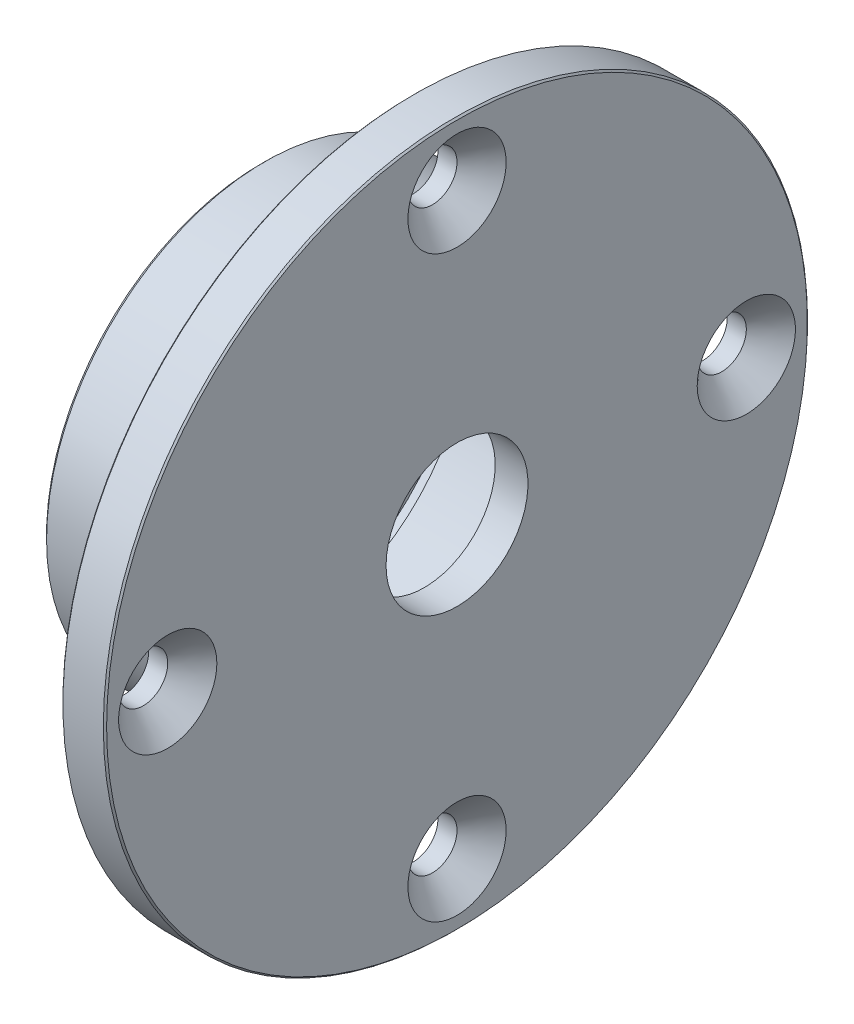
SolidWorks part; units mm, degrees
material "6063-T6"
ref_plane "Front Plane" through (0, 0, 0) normal (0, 0, 1) x (1, 0, 0)
ref_plane "Top Plane" through (0, 0, 0) normal (0, 1, 0) x (1, 0, 0)
ref_plane "Right Plane" through (0, 0, 0) normal (1, 0, 0) x (0, 0, -1)
sketch "Sketch1" plane through (0, 0, 0) normal (0, 0, 1) x (1, 0, 0)
  line L0 (0, 16) -> (1.6954, 16)
  line L1 (13, 16) -> (13, 12.5)
  line L2 (13, 12.5) -> (15, 12.5)
  line L3 (15, 12.5) -> (15, 0)
  line L4 (15, 0) -> (18, 0)
  line L5 (18, 0) -> (18, 32.5)
  line L6 (18, 32.5) -> (14, 32.5)
  line L7 (14, 32.5) -> (14, 20)
  line L8 (14, 20) -> (0, 20)
  line L9 (0, 20) -> (0, 16)
  line L10 (1.6954, 16) -> (1.6954, 16.85)
  line L11 (1.6954, 16.85) -> (2.9954, 16.85)
  line L12 (2.9954, 16.85) -> (2.9954, 16)
  line L13 (2.9954, 16) -> (13, 16)
  dimension "D1" = 16
  dimension "D2" = 2
  dimension "D3" = 12.5
  dimension "D4" = 18
  dimension "D5" = 4
  dimension "D6" = 3
  dimension "D7" = 20
  dimension "D8" = 32.5
  dimension "D9" = 1.3
  dimension "D10" = 16.85
  dimension "D11" = 10.0046
revolve "Revolve1" add sketch "Sketch1" angle 360 about L4
sketch "Sketch2" plane through (0, 0, 0) normal (0, 1, 0) x (1, 0, 0)
  line L0 (14, 26.5) -> (18, 26.5)
  line L1 (14, 32.5) -> (14, -32.5) construction
  line L2 (18, -32.5) -> (18, 32.5) construction
  line L3 (18, 26.5) -> (18, 31)
  line L4 (18, 31) -> (15.75, 28.75)
  line L5 (15.75, 28.75) -> (14, 28.75)
  line L6 (14, 28.75) -> (14, 26.5)
  dimension "D1" = 26.5
  dimension "D2" = 2.25
  dimension "D3" = 4.5
  dimension "D4" = 45
revolve "Cut-Revolve1" cut sketch "Sketch2" angle 360 about L0
pattern_circular "CirPattern1" count 4 over 360 about axis through (0, 0, 0) along (1, 0, 0) of "Cut-Revolve1"
chamfer "Chamfer1" distance 0.4 angle 45 5 edges at (13, 0, 12.5) (0, 0, 16) (18, 0, 32.5) (14, 0, 32.5) (0, 0, 20)
hole_wizard "M4 Tapped Hole1" positions "Sketch4" profile "Sketch5" tap size "M4" standard "GB"
sketch "Sketch4" plane through (18, 0, 0) normal (1, 0, 0) x (0, 0, -1)
  line L0 (0, 0) -> (26.5, 0) construction
  line L2 (0, 0) -> (10.0763, 10.0763) construction
  circle A0 centre (0, 0) radius 14.25
  point P13 (10.0763, 10.0763)
  dimension "D1" = 28.5
  dimension "D2" = 45
cosmetic thread "Hole thread1" [suppressed] parameters "D2"=4
sketch "Sketch5" plane through (18, 10.0763, -10.0763) normal (0, 1, 0) x (0, 0, -1)
  line L0 (0, 0) -> (0, 18)
  line L1 (0, 18) -> (1.65, 18)
  line L2 (1.65, 18) -> (1.65, 0)
  line L5 (1.65, 0) -> (0, 0)
  line L11 (0, -6.35) -> (0, 107.95) construction
  dimension "通孔螺纹孔钻头直径" = 3.3
  dimension "通孔螺纹孔钻头深度" = 18
pattern_circular "CirPattern2" [suppressed] count 2 over 360
sketch "Sketch8" plane through (15, 0, 0) normal (-1, 0, 0) x (0, 0, 1)
  circle A0 centre (0, 0) radius 6.5
  dimension "D1" = 13
extrude "Cut-Extrude1" cut sketch "Sketch8" against normal blind 10
sketch "Sketch9" plane through (18, 0, 0) normal (1, 0, 0) x (0, 0, -1)
  circle A0 centre (0, 0) radius 32.25
  circle A1 centre (0, 0) radius 33
  dimension "D1" = 64.5
  dimension "D2" = 66
extrude "Cut-Extrude2" cut sketch "Sketch9" against normal blind 10
